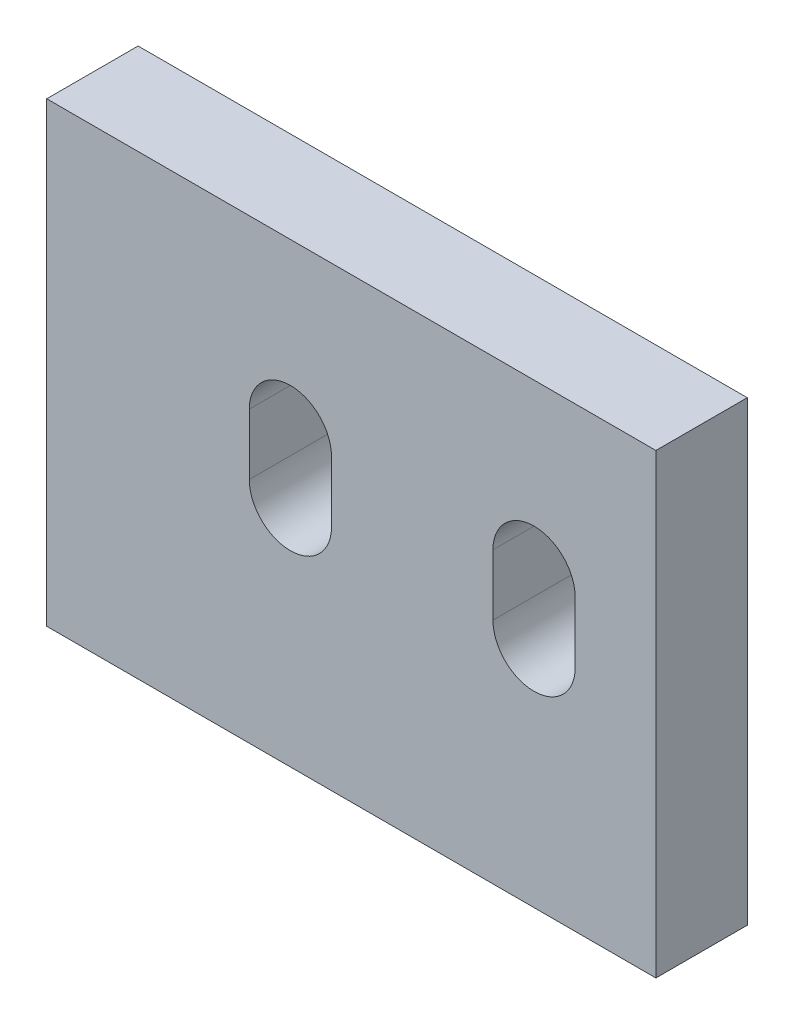
SolidWorks part; units mm, degrees
material "Q235B"
ref_plane "Front Plane" through (0, 0, 0) normal (0, 0, 1) x (1, 0, 0)
ref_plane "Top Plane" through (0, 0, 0) normal (0, 1, 0) x (1, 0, 0)
ref_plane "Right Plane" through (0, 0, 0) normal (1, 0, 0) x (0, 0, -1)
sketch "Sketch1" plane through (0, 0, 0) normal (0, 0, 1) x (1, 0, 0)
  line L0 (80, 95) -> (80, 75) construction
  line L1 (0, 0) -> (200, 0)
  line L2 (0, 0) -> (0, 150)
  line L3 (0, 150) -> (200, 150)
  line L4 (200, 0) -> (200, 150)
  line L5 (93.5, 95) -> (93.5, 75)
  line L6 (66.5, 95) -> (66.5, 75)
  line L7 (160, 95) -> (160, 75) construction
  line L8 (173.5, 95) -> (173.5, 75)
  line L9 (146.5, 95) -> (146.5, 75)
  arc A0 (93.5, 95) -> (66.5, 95) centre (80, 95) ccw
  arc A1 (66.5, 75) -> (93.5, 75) centre (80, 75) ccw
  arc A2 (173.5, 95) -> (146.5, 95) centre (160, 95) ccw
  arc A3 (146.5, 75) -> (173.5, 75) centre (160, 75) ccw
  point P7 (80, 85)
  point P12 (160, 85)
  dimension "D3" = 13.5
  dimension "D1" = 200
  dimension "D2" = 150
  dimension "D4" = 20
  dimension "D5" = 40
  dimension "D6" = 80
  dimension "D7" = 65
extrude "Boss-Extrude1" add sketch "Sketch1" along normal blind 30
